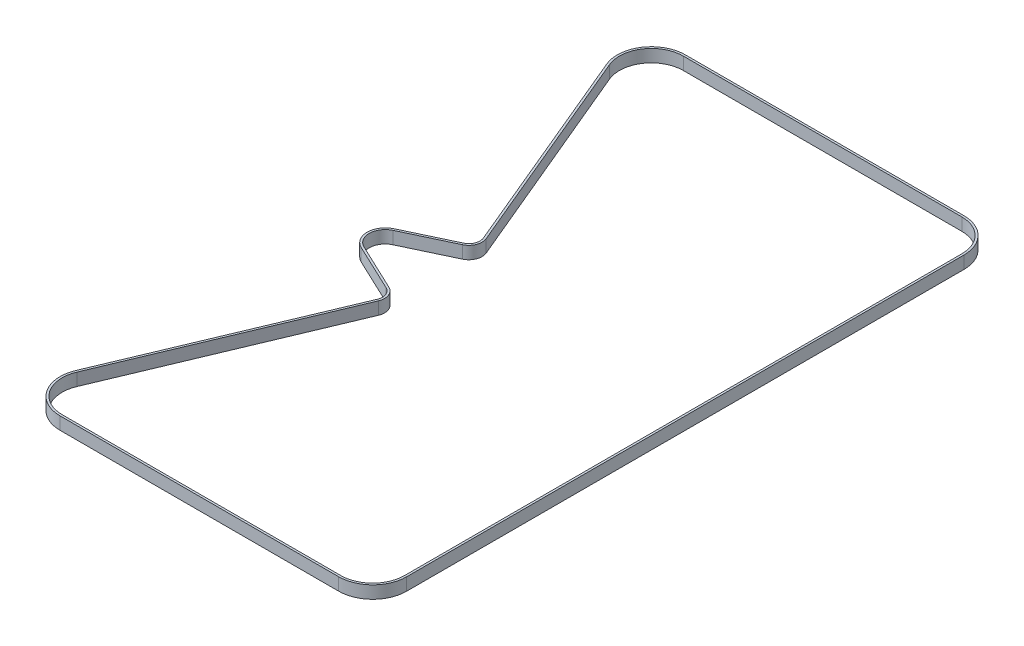
from build123d import *

# Parameters (mm, degrees)
BOSS_EXTRUDE1_DEPTH = 9


with BuildPart() as part:
    # Sketch1 → Boss-Extrude1 (new body)
    with BuildSketch(Plane(origin=(0, 0, 0), x_dir=(-1, 0, 0), z_dir=(0, 1, 0))):
        with BuildLine():
            Line((-145.613884922, 900), (-145.613884922, 500))
            ThreePointArc((-145.613884922, 500), (-138.461432518, 482.732452403), (-121.193884922, 475.58))
            Line((-121.193884922, 475.58), (78.806115078, 475.58))
            ThreePointArc((78.806115078, 475.58), (99.138824975, 486.475307462), (101.328117521, 509.439057473))
            Line((101.328117521, 509.439057473), (37.4278997, 661.90776168))
            ThreePointArc((37.4278997, 661.90776168), (37.336543074, 667.86452336), (41.387455782, 672.23275664))
            Line((41.387455782, 672.23275664), (75.344343138, 688.282934243))
            ThreePointArc((75.344343138, 688.282934243), (82.766115078, 700), (75.344343138, 711.717065757))
            Line((75.344343138, 711.717065757), (41.387455782, 727.76724336))
            ThreePointArc((41.387455782, 727.76724336), (37.336543074, 732.13547664), (37.4278997, 738.09223832))
            Line((37.4278997, 738.09223832), (101.328117521, 890.560942527))
            ThreePointArc((101.328117521, 890.560942527), (99.138824975, 913.524692538), (78.806115078, 924.42))
            Line((78.806115078, 924.42), (-121.193884922, 924.42))
            ThreePointArc((-121.193884922, 924.42), (-138.461432518, 917.267547597), (-145.613884922, 900))
        make_face()
        with BuildLine():
            Line((-144.113884922, 900), (-144.113884922, 500))
            ThreePointArc((-144.113884922, 500), (-137.400772347, 483.793112575), (-121.193884922, 477.08))
            Line((-121.193884922, 477.08), (78.806115078, 477.08))
            ThreePointArc((78.806115078, 477.08), (97.889887021, 487.306062532), (99.944702137, 508.859262788))
            Line((99.944702137, 508.859262788), (36.044484316, 661.327966995))
            ThreePointArc((36.044484316, 661.327966995), (35.935998324, 668.40162149), (40.746457164, 673.58889851))
            Line((40.746457164, 673.58889851), (74.70334452, 689.639076113))
            ThreePointArc((74.70334452, 689.639076113), (81.266115078, 700), (74.70334452, 710.360923887))
            Line((74.70334452, 710.360923887), (40.746457164, 726.41110149))
            ThreePointArc((40.746457164, 726.41110149), (35.935998324, 731.59837851), (36.044484316, 738.672033005))
            Line((36.044484316, 738.672033005), (99.944702137, 891.140737212))
            ThreePointArc((99.944702137, 891.140737212), (97.889887021, 912.693937468), (78.806115078, 922.92))
            Line((78.806115078, 922.92), (-121.193884922, 922.92))
            ThreePointArc((-121.193884922, 922.92), (-137.400772347, 916.206887425), (-144.113884922, 900))
        make_face(mode=Mode.SUBTRACT)
    extrude(amount=BOSS_EXTRUDE1_DEPTH)


solid = part.part
